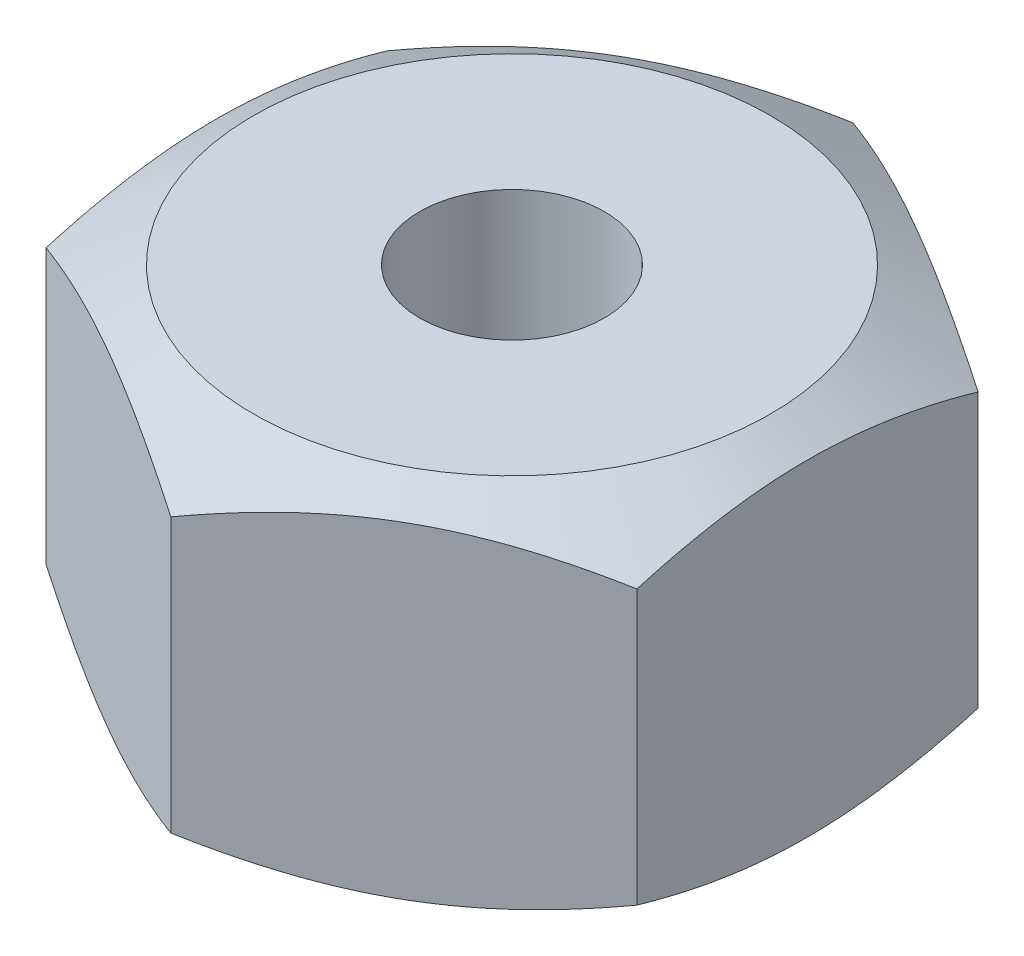
SolidWorks part; units mm, degrees
ref_plane "Front Plane" through (0, 0, 0) normal (0, 0, 1) x (1, 0, 0)
ref_plane "Top Plane" through (0, 0, 0) normal (0, 1, 0) x (1, 0, 0)
ref_plane "Right Plane" through (0, 0, 0) normal (1, 0, 0) x (0, 0, -1)
other "Configuration Table"
sketch "Sketch1" plane through (0, 0, 0) normal (0, 1, 0) x (1, 0, 0)
  line L1 (0, 18.4752) -> (-16, 9.2376)
  line L2 (-16, 9.2376) -> (-16, -9.2376)
  line L3 (-16, -9.2376) -> (0, -18.4752)
  line L4 (0, -18.4752) -> (16, -9.2376)
  line L5 (16, -9.2376) -> (16, 9.2376)
  line L6 (16, 9.2376) -> (0, 18.4752)
  circle A0 centre (0, 0) radius 16 construction
  dimension "D1" = 32
extrude "Boss-Extrude1" add sketch "Sketch1" along normal mid plane 20
sketch "Sketch2" plane through (0, 10, 0) normal (0, 1, 0) x (1, 0, 0)
  circle A0 centre (0, 0) radius 5
  dimension "D1" = 10
extrude "Cut-Extrude1" cut sketch "Sketch2" against normal blind 50
sketch "Sketch3" plane through (0, 10, 0) normal (0, 1, 0) x (1, 0, 0)
  circle A0 centre (0, 0) radius 14
  dimension "D1" = 28
extrude "Cut-Extrude2" cut sketch "Sketch3" along normal blind 4 from offset 15 offset against normal yes
sketch "Sketch4" plane through (0, 0, 0) normal (1, 0, 0) x (0, 0, -1)
  line L0 (0, 0) -> (0, 26.5652) construction
  line L1 (18.4752, 7.4162) -> (18.4752, 10)
  line L2 (18.4752, 10) -> (18.4752, -10) construction
  line L3 (18.4752, 10) -> (14, 10)
  line L4 (18.4752, 10) -> (9.2376, 10) construction
  line L5 (14, 10) -> (18.4752, 7.4162)
  dimension "D1" = 30
  dimension "D2" = 28
revolve "Cut-Revolve1" cut sketch "Sketch4" angle 360 about L0
mirror "Mirror1" about plane through (0, 0, 0) normal (0, 1, 0) of "Cut-Revolve1"
